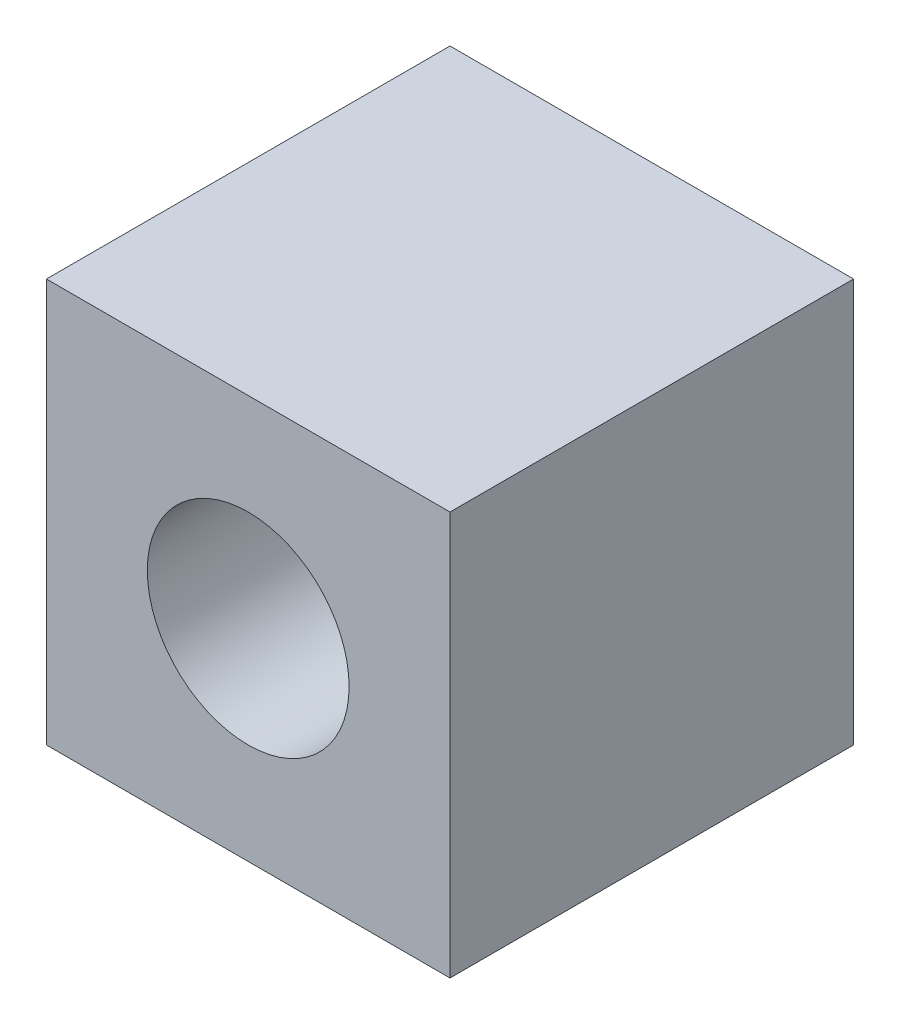
SolidWorks part; units mm, degrees
ref_plane "Plane1" through (0, 0, 0) normal (0, 0, 1) x (1, 0, 0)
ref_plane "Plane2" through (0, 0, 0) normal (0, 1, 0) x (1, 0, 0)
ref_plane "Plane3" through (0, 0, 0) normal (1, 0, 0) x (0, 0, -1)
sketch "Sketch1" plane through (0, 0, 0) normal (0, 0, 1) x (1, 0, 0)
  line L1 (10, 10) -> (-10, 10)
  line L2 (-10, 10) -> (-10, -10)
  line L3 (-10, -10) -> (10, -10)
  line L4 (10, -10) -> (10, 10)
  circle A0 centre (0, 0) radius 10 construction
extrude "Base-Extrude" add sketch "Sketch1" along normal blind 20
sketch "Sketch2" plane through (0, 0, 20) normal (0, 0, 1) x (1, 0, 0)
  circle A0 centre (0, 0) radius 5
  dimension "D1" = 10
extrude "Cut-Extrude1" cut sketch "Sketch2" against normal through all
